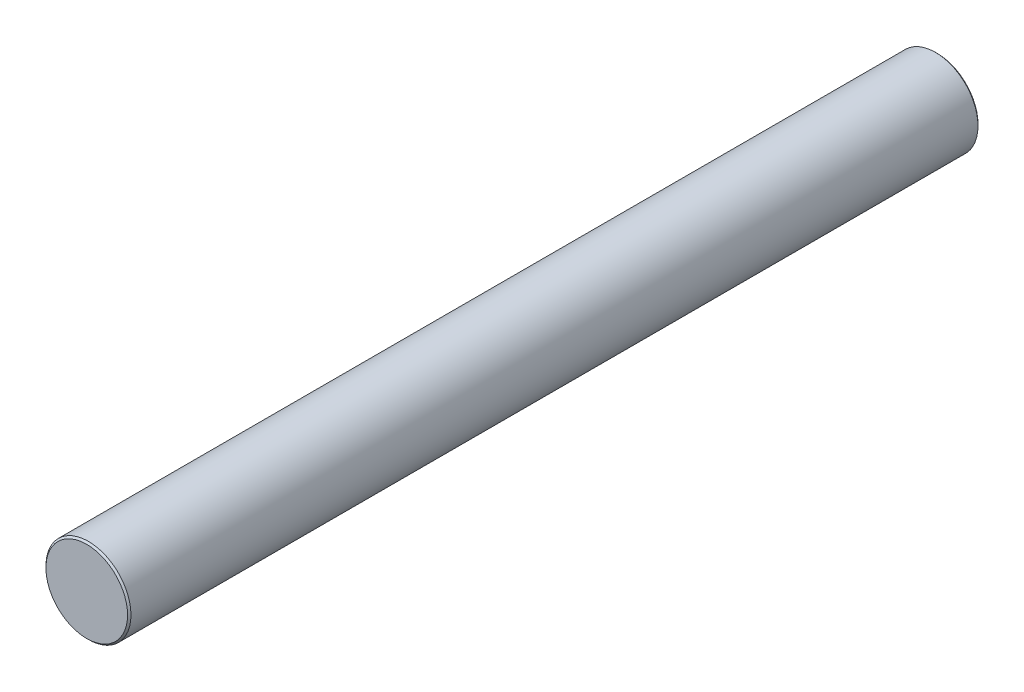
SolidWorks part; units mm, degrees
ref_plane "Front Plane" through (0, 0, 0) normal (0, 0, 1) x (1, 0, 0)
ref_plane "Top Plane" through (0, 0, 0) normal (0, 1, 0) x (1, 0, 0)
ref_plane "Right Plane" through (0, 0, 0) normal (1, 0, 0) x (0, 0, -1)
other "Configuration Table"
sketch "Sketch1" plane through (0, 0, 0) normal (0, 0, 1) x (1, 0, 0)
  circle A0 centre (0, 0) radius 2.5
  dimension "D1" = 5
extrude "Boss-Extrude1" add sketch "Sketch1" along normal mid plane 50 contours A0
chamfer "Chamfer1" distance 0.1 angle 45 2 edges at (2.5, 0, 25) (2.5, 0, -25)
